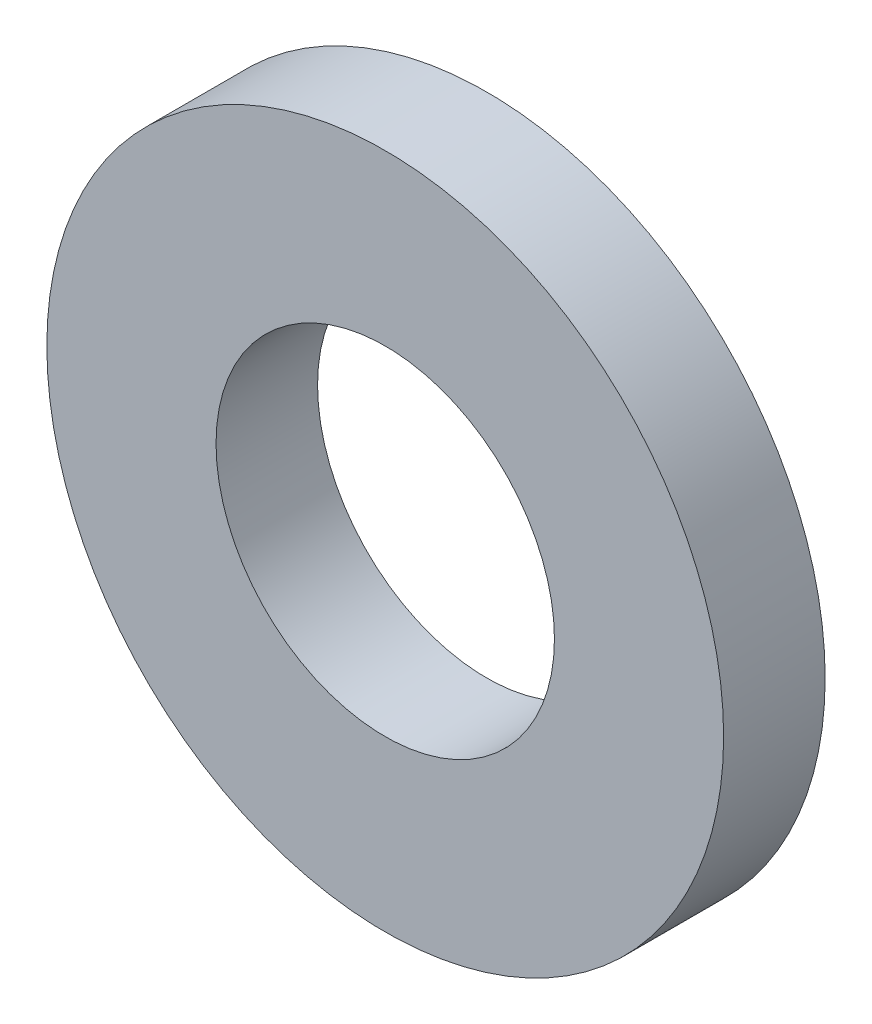
SolidWorks part; units mm, degrees
ref_plane "Front Plane" through (0, 0, 0) normal (0, 0, 1) x (1, 0, 0)
ref_plane "Top Plane" through (0, 0, 0) normal (0, 1, 0) x (1, 0, 0)
ref_plane "Right Plane" through (0, 0, 0) normal (1, 0, 0) x (0, 0, -1)
sketch "Sketch1" plane through (0, 0, 0) normal (0, 0, 1) x (1, 0, 0)
  circle A0 centre (0, 0) radius 5
  circle A1 centre (0, 0) radius 2.5
  dimension "D1" = 10
  dimension "D2" = 5
extrude "Boss-Extrude1" add sketch "Sketch1" along normal blind 1.5
